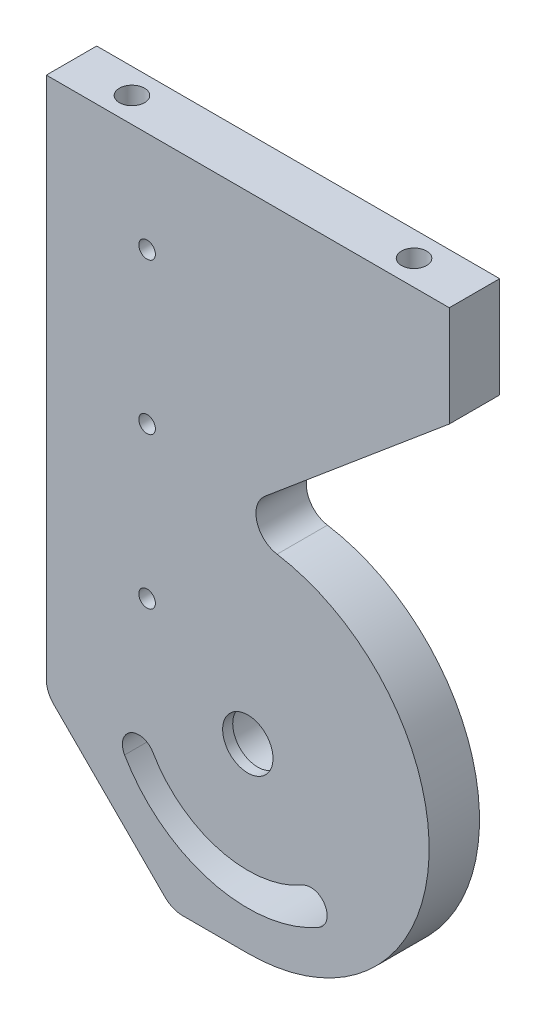
from build123d import *

# Parameters (mm, degrees)
SKETCH_1_W                = 80
SKETCH_1_H                = 170
EXTRUDE_1_DEPTH           = 5
HOLE_WIZARD_1_D           = 10
HOLE_WIZARD_1_CBORE_D     = 12
HOLE_WIZARD_1_CBORE_DEPTH = 8
CUT_EXTRUDE_2_DEPTH       = 95.472218138
CUT_EXTRUDE_4_DEPTH       = 95.472218138
FILLET_1_R                = 5
HOLE_WIZARD_M6_1_D        = 5
HOLE_WIZARD_M6_1_DEPTH    = 17
HOLE_WIZARD_M6_1_TIP      = 1.502151548
HOLE_WIZARD_M4_1_D        = 3.3


with BuildPart() as part:
    # 草图1 → 凸台-拉伸1 (new, symmetric)
    with BuildSketch(Plane.XY):
        Rectangle(SKETCH_1_W, SKETCH_1_H)
    extrude(amount=EXTRUDE_1_DEPTH, both=True)

    # 孔1 (through all)
    with Locations(Plane(origin=(0, 0, -5), x_dir=(-1, 0, 0), z_dir=(0, 0, -1))):
        with Locations((0, -10)):
            CounterBoreHole(HOLE_WIZARD_1_D / 2, HOLE_WIZARD_1_CBORE_D / 2, HOLE_WIZARD_1_CBORE_DEPTH)

    # 草图6 → 切除-拉伸2 (cut, through all)
    with BuildSketch(Plane(origin=(0, 0, -5), x_dir=(-1, 0, 0), z_dir=(0, 0, -1))):
        with BuildLine():
            ThreePointArc((-14.125, -34.465217657), (7.311638024, -37.287404593), (24.465217657, -24.125))
            ThreePointArc((24.465217657, -24.125), (23.275635095, -19.685417438), (18.836052532, -20.875))
            ThreePointArc((18.836052532, -20.875), (5.629314231, -31.008886722), (-10.875, -28.836052532))
            ThreePointArc((-10.875, -28.836052532), (-15.314582562, -30.025635095), (-14.125, -34.465217657))
        make_face()
    extrude(amount=-CUT_EXTRUDE_2_DEPTH, mode=Mode.SUBTRACT)

    # 草图11 → 切除-拉伸4 (cut, through all)
    with BuildSketch(Plane(origin=(0, 0, -5), x_dir=(-1, 0, 0), z_dir=(0, 0, -1))):
        with BuildLine():
            Line((0, -46), (15, -46))
            Line((15, -46), (40, -21))
            Line((40, -21), (40, -85))
            Line((40, -85), (-40, -85))
            Line((-40, -85), (-40, 65))
            Line((-40, 65), (7.392754444, 25.232757226))
            ThreePointArc((7.392754444, 25.232757226), (-35.807675575, -6.283769392), (0, -46))
        make_face()
    extrude(amount=-CUT_EXTRUDE_4_DEPTH, mode=Mode.SUBTRACT)

    # 圆角1
    fillet_1_edges = [part.edges().sort_by_distance(p)[0] for p in [
        (-40, -21, 0),
        (-7.392754444, 25.232757226, 0),
        (-15, -46, 0),
    ]]
    fillet(fillet_1_edges, radius=FILLET_1_R)

    # M6 螺纹孔1
    with Locations(Plane(origin=(0, 85, 0), x_dir=(1, 0, 0), z_dir=(0, 1, 0))):
        with Locations((-28, 0), (28, 0)):
            Hole(HOLE_WIZARD_M6_1_D / 2, depth=HOLE_WIZARD_M6_1_DEPTH)
            with Locations((0, 0, -(HOLE_WIZARD_M6_1_DEPTH + HOLE_WIZARD_M6_1_TIP / 2))):  # 118° drill point
                Cone(0, HOLE_WIZARD_M6_1_D / 2, HOLE_WIZARD_M6_1_TIP, mode=Mode.SUBTRACT)

    # M4 螺纹孔1 (through all)
    with Locations(Plane.XY.offset(5)):
        with Locations((-20, 65), (-20, 35), (-20, 5)):
            Hole(HOLE_WIZARD_M4_1_D / 2)


solid = part.part
